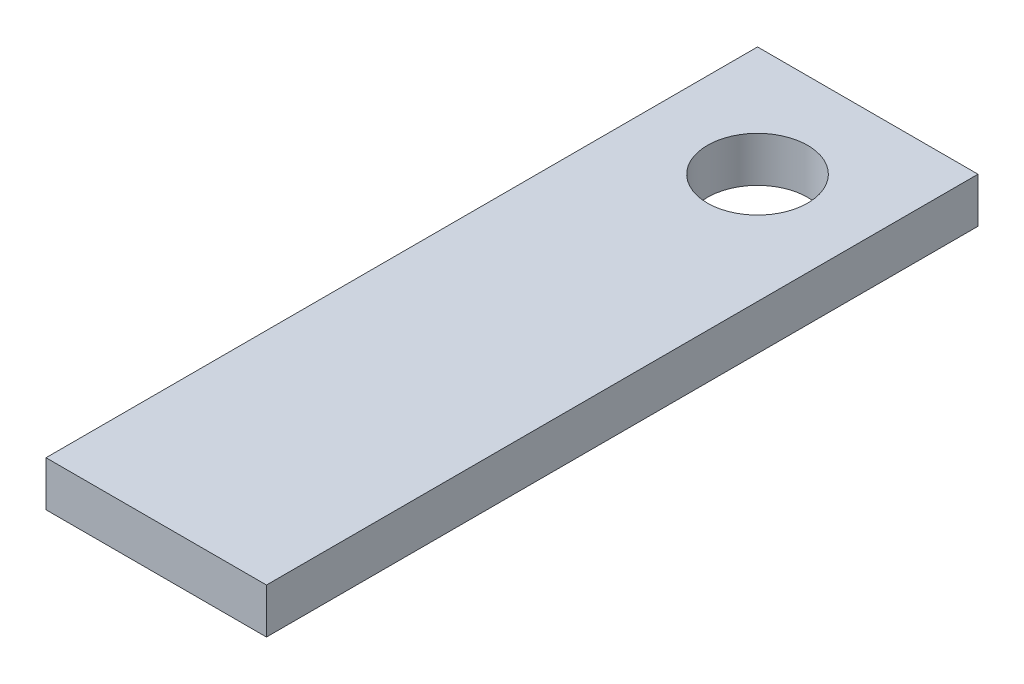
from build123d import *

# Parameters (mm, degrees)
SKETCH1_W           = 22
SKETCH1_H           = 71
SKETCH1_R           = 5
BOSS_EXTRUDE1_DEPTH = 4.5


with BuildPart() as part:
    # Sketch1 → Boss-Extrude1 (new body)
    with BuildSketch(Plane(origin=(0, 0, 0), x_dir=(1, 0, 0), z_dir=(0, 1, 0))):
        with Locations((11, 35.5)):
            Rectangle(SKETCH1_W, SKETCH1_H)
        with Locations(Location((11, 60, 0), (0, 0, 270))):
            Circle(SKETCH1_R, mode=Mode.SUBTRACT)
    extrude(amount=BOSS_EXTRUDE1_DEPTH)


solid = part.part
